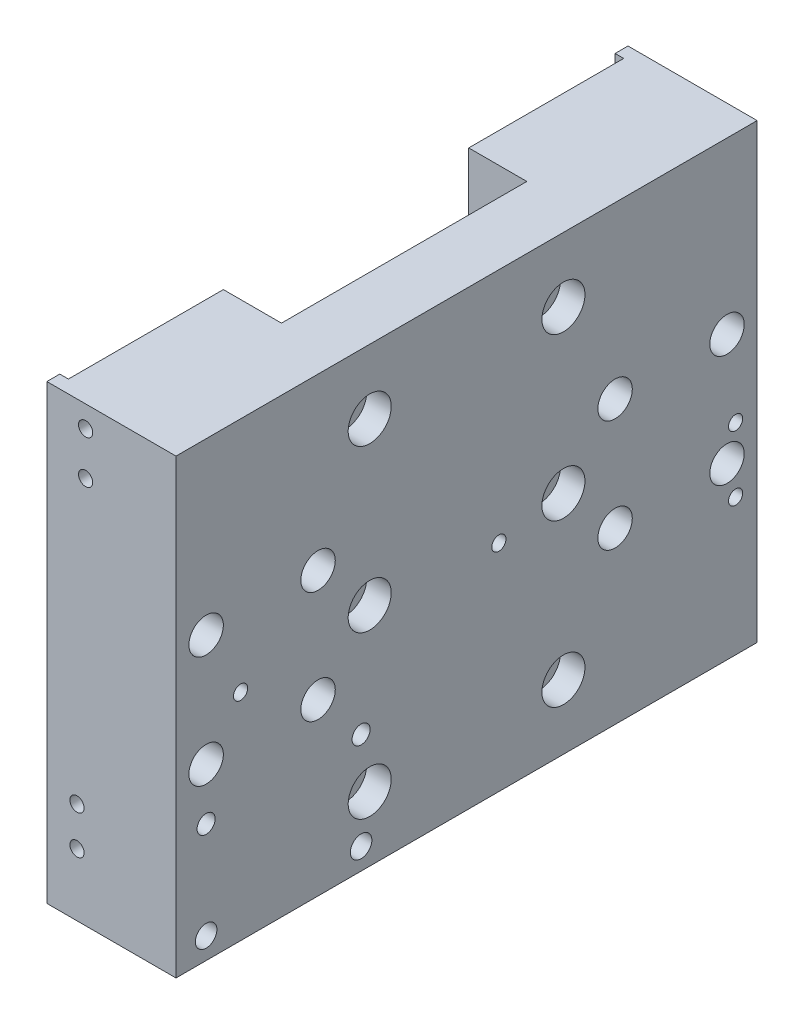
from build123d import *

# Parameters (mm, degrees)
SKETCH1_W                                            = 135
SKETCH1_H                                            = 105
BOSS_EXTRUDE1_DEPTH                                  = 30
SKETCH2_W                                            = 15.5
SKETCH2_H                                            = 57
CUT_EXTRUDE1_DEPTH                                   = 129.379320765
SKETCH3_W                                            = 129
SKETCH3_H                                            = 105
CUT_EXTRUDE2_DEPTH                                   = 2
CBORE_FOR_M5_HEXAGON_SOCKET_HEAD_CAP_SCR_D           = 5.5
CBORE_FOR_M5_HEXAGON_SOCKET_HEAD_CAP_SCR_CBORE_D     = 10
CBORE_FOR_M5_HEXAGON_SOCKET_HEAD_CAP_SCR_CBORE_DEPTH = 5.7
CBORE_FOR_M4_HEXAGON_SOCKET_HEAD_CAP_SCR_D           = 4.5
CBORE_FOR_M4_HEXAGON_SOCKET_HEAD_CAP_SCR_CBORE_D     = 8
CBORE_FOR_M4_HEXAGON_SOCKET_HEAD_CAP_SCR_CBORE_DEPTH = 23
M4_TAPPED_HOLE1_D                                    = 3.3
M4_TAPPED_HOLE1_DEPTH                                = 10.1
M4_TAPPED_HOLE1_TIP                                  = 0.991420021
M6_TAPPED_HOLE1_D                                    = 5
M6_TAPPED_HOLE1_DEPTH                                = 15
M6_TAPPED_HOLE1_TIP                                  = 1.502151548
M4_TAPPED_HOLE2_D                                    = 3.3
M4_TAPPED_HOLE2_DEPTH                                = 10.1
M4_TAPPED_HOLE2_TIP                                  = 0.991420021
M4_TAPPED_HOLE3_D                                    = 3.3
M4_TAPPED_HOLE3_DEPTH                                = 10.1
M4_TAPPED_HOLE3_TIP                                  = 0.991420021
M5_TAPPED_HOLE1_D                                    = 4.2
M5_TAPPED_HOLE1_DEPTH                                = 12.4
M5_TAPPED_HOLE1_TIP                                  = 1.2618073
F_5_0MM_DOWEL_HOLE1_D                                = 5
F_5_0MM_DOWEL_HOLE1_DEPTH                            = 6
F_5_0MM_DOWEL_HOLE1_TIP                              = 1.502151548
M4_TAPPED_HOLE4_D                                    = 3.3
M4_TAPPED_HOLE4_DEPTH                                = 10.1
M4_TAPPED_HOLE4_TIP                                  = 0.991420021


with BuildPart() as part:
    # Sketch1 → Boss-Extrude1 (new body)
    with BuildSketch(Plane(origin=(0, 0, 0), x_dir=(0, 0, -1), z_dir=(1, 0, 0))):
        Rectangle(SKETCH1_W, SKETCH1_H)
    extrude(amount=BOSS_EXTRUDE1_DEPTH)

    # Sketch2 → Cut-Extrude1 (cut, through all)
    with BuildSketch(Plane.XZ.offset(52.5)):
        with Locations((7.75, 0)):
            Rectangle(SKETCH2_W, SKETCH2_H)
    extrude(amount=-CUT_EXTRUDE1_DEPTH, mode=Mode.SUBTRACT)

    # Sketch3 → Cut-Extrude2 (cut)
    with BuildSketch(Plane.ZY):
        Rectangle(SKETCH3_W, SKETCH3_H)
    extrude(amount=-CUT_EXTRUDE2_DEPTH, mode=Mode.SUBTRACT)

    # CBORE for M5 Hexagon socket head cap screws1 (through all)
    with Locations(Plane(origin=(30, 0, 0), x_dir=(0, 0, -1), z_dir=(1, 0, 0))):
        with Locations((22.5, -37.5), (22.5, 37.5), (-22.5, 37.5), (-22.5, 0), (22.5, 0), (-22.5, -37.5)):
            CounterBoreHole(CBORE_FOR_M5_HEXAGON_SOCKET_HEAD_CAP_SCR_D / 2, CBORE_FOR_M5_HEXAGON_SOCKET_HEAD_CAP_SCR_CBORE_D / 2, CBORE_FOR_M5_HEXAGON_SOCKET_HEAD_CAP_SCR_CBORE_DEPTH)

    # CBORE for M4 Hexagon socket head cap screws1 (through all)
    with Locations(Plane(origin=(30, 0, 0), x_dir=(0, 0, -1), z_dir=(1, 0, 0))):
        with Locations((34.5, 13), (60.5, 13), (60.5, -13), (34.5, -13)):
            cbore_for_m4_hexagon_socket_head_cap_scr = CounterBoreHole(CBORE_FOR_M4_HEXAGON_SOCKET_HEAD_CAP_SCR_D / 2, CBORE_FOR_M4_HEXAGON_SOCKET_HEAD_CAP_SCR_CBORE_D / 2, CBORE_FOR_M4_HEXAGON_SOCKET_HEAD_CAP_SCR_CBORE_DEPTH)

    # Mirror1: CBORE for M4 Hexagon socket head cap screws1 across plane
    add(cbore_for_m4_hexagon_socket_head_cap_scr.mirror(Plane.XY), mode=Mode.SUBTRACT)

    # M4 Tapped Hole1
    with Locations(Plane(origin=(30, 0, 0), x_dir=(0, 0, -1), z_dir=(1, 0, 0))):
        with Locations((62.5, -5.75), (62.5, -20.75)):
            Hole(M4_TAPPED_HOLE1_D / 2, depth=M4_TAPPED_HOLE1_DEPTH)
            with Locations((0, 0, -(M4_TAPPED_HOLE1_DEPTH + M4_TAPPED_HOLE1_TIP / 2))):  # 118° drill point
                Cone(0, M4_TAPPED_HOLE1_D / 2, M4_TAPPED_HOLE1_TIP, mode=Mode.SUBTRACT)

    # M6 Tapped Hole1
    with Locations(Plane(origin=(0, 0, -67.5), x_dir=(-1, 0, 0), z_dir=(0, 0, -1))):
        with Locations((-12, 42.5), (-12, 22.5)):
            Hole(M6_TAPPED_HOLE1_D / 2, depth=M6_TAPPED_HOLE1_DEPTH)
            with Locations((0, 0, -(M6_TAPPED_HOLE1_DEPTH + M6_TAPPED_HOLE1_TIP / 2))):  # 118° drill point
                Cone(0, M6_TAPPED_HOLE1_D / 2, M6_TAPPED_HOLE1_TIP, mode=Mode.SUBTRACT)

    # M4 Tapped Hole2
    with Locations(Plane.XY.offset(67.5)):
        with Locations((9, 37.5), (9, 47.5)):
            Hole(M4_TAPPED_HOLE2_D / 2, depth=M4_TAPPED_HOLE2_DEPTH)
            with Locations((0, 0, -(M4_TAPPED_HOLE2_DEPTH + M4_TAPPED_HOLE2_TIP / 2))):  # 118° drill point
                Cone(0, M4_TAPPED_HOLE2_D / 2, M4_TAPPED_HOLE2_TIP, mode=Mode.SUBTRACT)

    # M4 Tapped Hole3
    with Locations(Plane.XY.offset(67.5)):
        with Locations((7, -29), (7, -38)):
            Hole(M4_TAPPED_HOLE3_D / 2, depth=M4_TAPPED_HOLE3_DEPTH)
            with Locations((0, 0, -(M4_TAPPED_HOLE3_DEPTH + M4_TAPPED_HOLE3_TIP / 2))):  # 118° drill point
                Cone(0, M4_TAPPED_HOLE3_D / 2, M4_TAPPED_HOLE3_TIP, mode=Mode.SUBTRACT)

    # M5 Tapped Hole1
    with Locations(Plane(origin=(30, 0, 0), x_dir=(0, 0, -1), z_dir=(1, 0, 0))):
        with Locations((-24.5, -25), (-60.5, -25)):
            Hole(M5_TAPPED_HOLE1_D / 2, depth=M5_TAPPED_HOLE1_DEPTH)
            with Locations((0, 0, -(M5_TAPPED_HOLE1_DEPTH + M5_TAPPED_HOLE1_TIP / 2))):  # 118° drill point
                Cone(0, M5_TAPPED_HOLE1_D / 2, M5_TAPPED_HOLE1_TIP, mode=Mode.SUBTRACT)

    # Ø5.0mm Dowel Hole1
    with Locations(Plane(origin=(30, 0, 0), x_dir=(0, 0, -1), z_dir=(1, 0, 0))):
        with Locations((-24.5, -47.5), (-60.5, -47.5)):
            Hole(F_5_0MM_DOWEL_HOLE1_D / 2, depth=F_5_0MM_DOWEL_HOLE1_DEPTH)
            with Locations((0, 0, -(F_5_0MM_DOWEL_HOLE1_DEPTH + F_5_0MM_DOWEL_HOLE1_TIP / 2))):  # 118° drill point
                Cone(0, F_5_0MM_DOWEL_HOLE1_D / 2, F_5_0MM_DOWEL_HOLE1_TIP, mode=Mode.SUBTRACT)

    # M4 Tapped Hole4
    with Locations(Plane(origin=(30, 0, 0), x_dir=(0, 0, -1), z_dir=(1, 0, 0))):
        with Locations((7.5, -2.5), (-52.5, -2.5)):
            Hole(M4_TAPPED_HOLE4_D / 2, depth=M4_TAPPED_HOLE4_DEPTH)
            with Locations((0, 0, -(M4_TAPPED_HOLE4_DEPTH + M4_TAPPED_HOLE4_TIP / 2))):  # 118° drill point
                Cone(0, M4_TAPPED_HOLE4_D / 2, M4_TAPPED_HOLE4_TIP, mode=Mode.SUBTRACT)


solid = part.part
